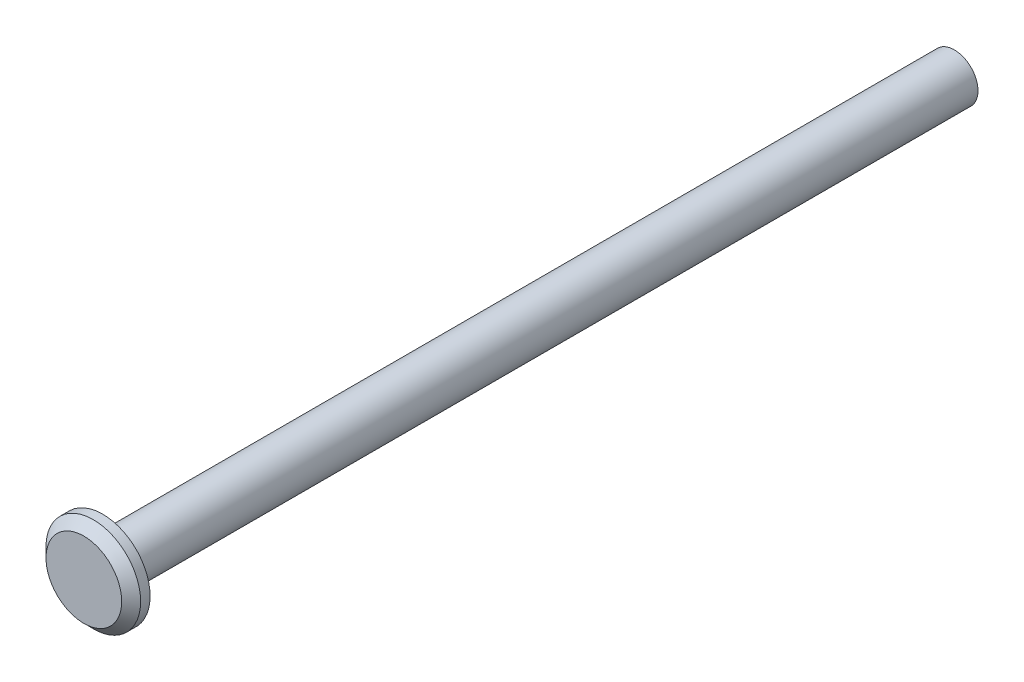
SolidWorks part; units mm, degrees
ref_plane "Front Plane" through (0, 0, 0) normal (0, 0, 1) x (1, 0, 0)
ref_plane "Top Plane" through (0, 0, 0) normal (0, 1, 0) x (1, 0, 0)
ref_plane "Right Plane" through (0, 0, 0) normal (1, 0, 0) x (0, 0, -1)
sketch "Sketch1" plane through (0, 0, 0) normal (0, 0, 1) x (1, 0, 0)
  circle A0 centre (0, 0) radius 2.5
  dimension "D1" = 5
extrude "Boss-Extrude1" add sketch "Sketch1" along normal blind 2 and the other way blind 90
sketch "Sketch2" plane through (0, 0, 2) normal (0, 0, 1) x (1, 0, 0)
  circle A0 centre (0, 0) radius 5
  dimension "D1" = 10
extrude "Boss-Extrude2" add sketch "Sketch2" against normal blind 2
chamfer "Chamfer1" distance 1 angle 45 1 edges at (5, 0, 2)
